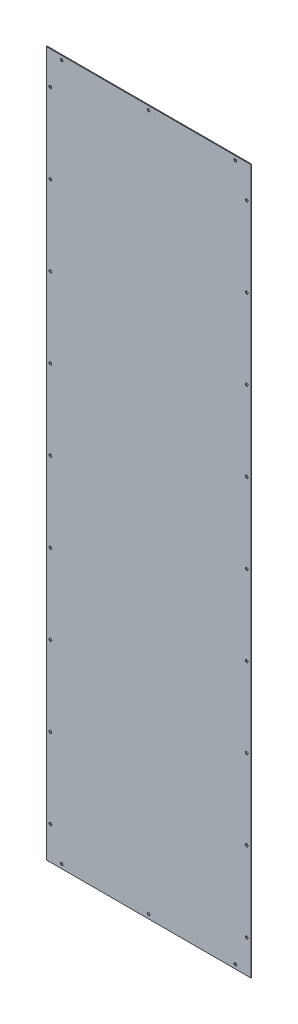
from build123d import *

# Parameters (mm, degrees)
SKETCH_1_W      = 494.5
SKETCH_1_H      = 1703
SKETCH_1_R      = 3.25
EXTRUDE_1_DEPTH = 2


with BuildPart() as part:
    # 草图1 → 凸台-拉伸1 (new body)
    with BuildSketch(Plane.XY):
        Rectangle(SKETCH_1_W, SKETCH_1_H)
        with Locations((-237.25, 0)):
            Circle(SKETCH_1_R, mode=Mode.SUBTRACT)
        with Locations((-237.25, -192.875)):
            Circle(SKETCH_1_R, mode=Mode.SUBTRACT)
        with Locations((-237.25, -385.75)):
            Circle(SKETCH_1_R, mode=Mode.SUBTRACT)
        with Locations((-237.25, -578.625)):
            Circle(SKETCH_1_R, mode=Mode.SUBTRACT)
        with Locations((-237.25, -771.5)):
            Circle(SKETCH_1_R, mode=Mode.SUBTRACT)
        with Locations((0, -841.5)):
            Circle(SKETCH_1_R, mode=Mode.SUBTRACT)
        with Locations(Location((0, 841.5, 0), (0, 0, 180))):
            Circle(SKETCH_1_R, mode=Mode.SUBTRACT)
        with Locations(Location((-237.25, 771.5, 0), (0, 0, 180))):
            Circle(SKETCH_1_R, mode=Mode.SUBTRACT)
        with Locations(Location((-237.25, 578.625, 0), (0, 0, 180))):
            Circle(SKETCH_1_R, mode=Mode.SUBTRACT)
        with Locations(Location((-237.25, 385.75, 0), (0, 0, 180))):
            Circle(SKETCH_1_R, mode=Mode.SUBTRACT)
        with Locations(Location((-237.25, 192.875, 0), (0, 0, 180))):
            Circle(SKETCH_1_R, mode=Mode.SUBTRACT)
        with Locations((237.25, 192.875)):
            Circle(SKETCH_1_R, mode=Mode.SUBTRACT)
        with Locations((237.25, 385.75)):
            Circle(SKETCH_1_R, mode=Mode.SUBTRACT)
        with Locations((237.25, 578.625)):
            Circle(SKETCH_1_R, mode=Mode.SUBTRACT)
        with Locations((237.25, 771.5)):
            Circle(SKETCH_1_R, mode=Mode.SUBTRACT)
        with Locations(Location((237.25, -771.5, 0), (0, 0, 180))):
            Circle(SKETCH_1_R, mode=Mode.SUBTRACT)
        with Locations(Location((237.25, -578.625, 0), (0, 0, 180))):
            Circle(SKETCH_1_R, mode=Mode.SUBTRACT)
        with Locations(Location((237.25, -385.75, 0), (0, 0, 180))):
            Circle(SKETCH_1_R, mode=Mode.SUBTRACT)
        with Locations(Location((237.25, -192.875, 0), (0, 0, 180))):
            Circle(SKETCH_1_R, mode=Mode.SUBTRACT)
        with Locations(Location((237.25, 0, 0), (0, 0, 180))):
            Circle(SKETCH_1_R, mode=Mode.SUBTRACT)
        with Locations((-210, 841.5)):
            Circle(SKETCH_1_R, mode=Mode.SUBTRACT)
        with Locations((210, 841.5)):
            Circle(SKETCH_1_R, mode=Mode.SUBTRACT)
        with Locations(Location((-210, -841.5, 0), (0, 0, 180))):
            Circle(SKETCH_1_R, mode=Mode.SUBTRACT)
        with Locations(Location((210, -841.5, 0), (0, 0, 180))):
            Circle(SKETCH_1_R, mode=Mode.SUBTRACT)
    extrude(amount=EXTRUDE_1_DEPTH)


solid = part.part
